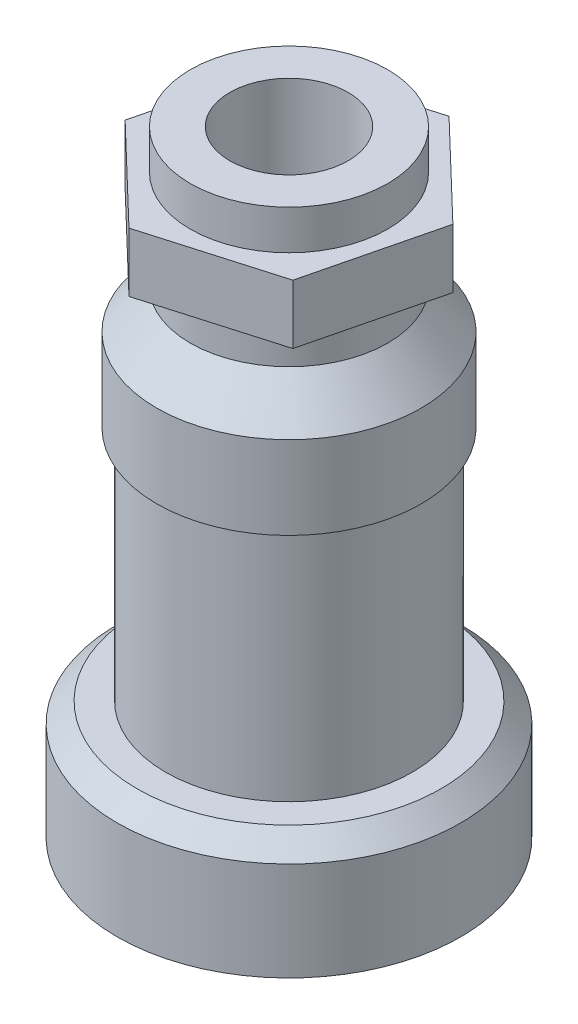
from build123d import *

# Parameters (mm, degrees)
BOSS_EXTRUDE1_DEPTH = 3
SKETCH3_R           = 3
CUT_EXTRUDE1_DEPTH  = 34.538336274
CHAMFER1_SIZE       = 1


with BuildPart() as part:
    # Sketch1 → Revolve1 (revolve)
    with BuildSketch(Plane.XY, mode=Mode.PRIVATE) as revolve1_sk:
        Polygon((0, 0), (5, 0), (5, -7), (6.7, -9), (6.7, -13.2), (6.25, -13.2), (6.25, -25.2), (8.7, -25.2), (8.7, -31.2), (0, -31.2), align=None)
    revolve(revolve1_sk.sketch.rotate(Axis((0, 0, 0), (0, -1, 0)), 90), axis=Axis((0, 0, 0), (0, -1, 0)))

    # Sketch2 → Boss-Extrude1 (add)
    with BuildSketch(Plane(origin=(0, -2, 0), x_dir=(1, 0, 0), z_dir=(0, 1, 0))):
        Polygon((-1.600084835, -6.506130073), (4.834431506, -4.638779152), (6.434516341, 1.867350921), (1.600084835, 6.506130073), (-4.834431506, 4.638779152), (-6.434516341, -1.867350921), align=None)
    extrude(amount=-BOSS_EXTRUDE1_DEPTH)

    # Sketch3 → Cut-Extrude1 (cut, through all)
    with BuildSketch(Plane(origin=(0, 0, 0), x_dir=(1, 0, 0), z_dir=(0, 1, 0))):
        with Locations(Location((0, 0, 0), (0, 0, 270))):
            Circle(SKETCH3_R)
    extrude(amount=-CUT_EXTRUDE1_DEPTH, mode=Mode.SUBTRACT)

    # Chamfer1
    chamfer1_edges = [part.edges().sort_by_distance(p)[0] for p in [
        (0, -25.2, -8.7),
    ]]
    chamfer(chamfer1_edges, length=CHAMFER1_SIZE)


solid = part.part
